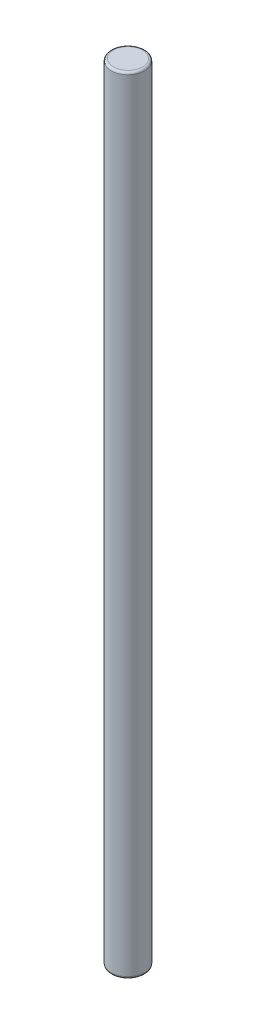
from build123d import *

# Parameters (mm, degrees)
SKETCH1_R           = 1.5
BOSS_EXTRUDE1_DEPTH = 70
FILLET1_R           = 0.2


with BuildPart() as part:
    # Sketch1 → Boss-Extrude1 (new body)
    with BuildSketch(Plane(origin=(0, 0, 0), x_dir=(1, 0, 0), z_dir=(0, 1, 0))):
        with Locations(Location((0, 0, 0), (0, 0, 270))):
            Circle(SKETCH1_R)
    extrude(amount=BOSS_EXTRUDE1_DEPTH)

    # Fillet1
    fillet1_edges = [part.edges().sort_by_distance(p)[0] for p in [
        (0, 0, -1.5),
        (0, 70, -1.5),
    ]]
    fillet(fillet1_edges, radius=FILLET1_R)


solid = part.part
